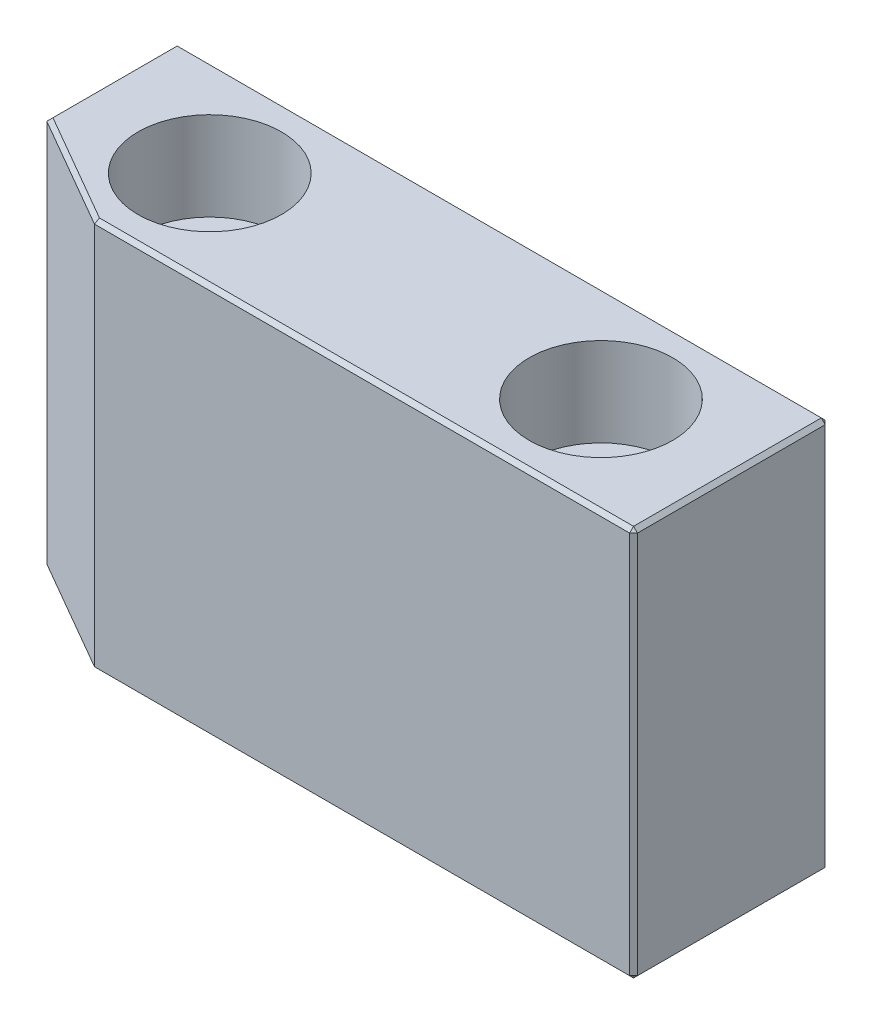
SolidWorks part; units mm, degrees
material "45号钢"
ref_plane "Front" through (0, 0, 0) normal (0, 0, 1) x (1, 0, 0)
ref_plane "Top" through (0, 0, 0) normal (0, 1, 0) x (1, 0, 0)
ref_plane "Right" through (0, 0, 0) normal (1, 0, 0) x (0, 0, -1)
sketch "草图1" plane through (0, 0, 0) normal (0, 0, 1) x (1, 0, 0)
  line L1 (-25, 15) -> (25, 15)
  line L2 (-25, 15) -> (-25, -15)
  line L3 (-25, -15) -> (25, -15)
  line L4 (25, 15) -> (25, -15)
  line L5 (-25, 15) -> (25, -15) construction
  line L6 (-25, -15) -> (25, 15) construction
  point P0 (0, 0)
  dimension "D1" = 50
  dimension "D2" = 30
extrude "凸台-拉伸1" add sketch "草图1" along normal blind 15
hole_wizard "打孔尺寸根据内六角圆柱头螺钉的类型1" positions "草图3" profile "草图2" counterbore size "M6" standard "Gb" end condition through all
sketch "草图3" plane through (0, 15, 0) normal (0, 1, 0) x (1, 0, 0)
  line L0 (25, -7.5) -> (15, -7.5) construction
  line L1 (25, -15) -> (25, 0) construction
  line L3 (0, 0) -> (0, -15) construction
  line L4 (25, -15) -> (-25, -15) construction
  point P0 (-15, -7.5)
  point P2 (15, -7.5)
  dimension "D1" = 30
sketch "草图2" plane through (-15, 15, 7.5) normal (1, 0, 0) x (0, 0, 1)
  line L0 (0, 0) -> (0, 30)
  line L1 (0, 30) -> (3.3, 30)
  line L3 (3.3, 30) -> (3.3, 6.8)
  line L4 (3.3, 6.8) -> (5.5, 6.8)
  line L5 (5.5, 6.8) -> (5.5, 0)
  line L7 (5.5, 0) -> (0, 0)
  line L11 (0, -6.35) -> (0, 107.95) construction
  dimension "通孔孔直径" = 6.6
  dimension "通孔孔深度" = 30
  dimension "柱形沉头孔直径" = 11
  dimension "柱形沉头孔深度" = 6.8
chamfer "倒角1" distance 5 angle 60 1 edges at (-25, 0, 15)
chamfer "倒角2" distance 0.3 angle 45 13 edges at (25, -15, 7.5) (25, 0, 15) (25, 15, 7.5) (0, 15, 0) (4.3301, 15, 15) (-20.6699, 15, 12.5) (-25, 15, 5) (-25, 0, 0) (25, 0, 0) (0, -15, 0) (4.3301, -15, 15) (-20.6699, -15, 12.5) (-25, -15, 5)
